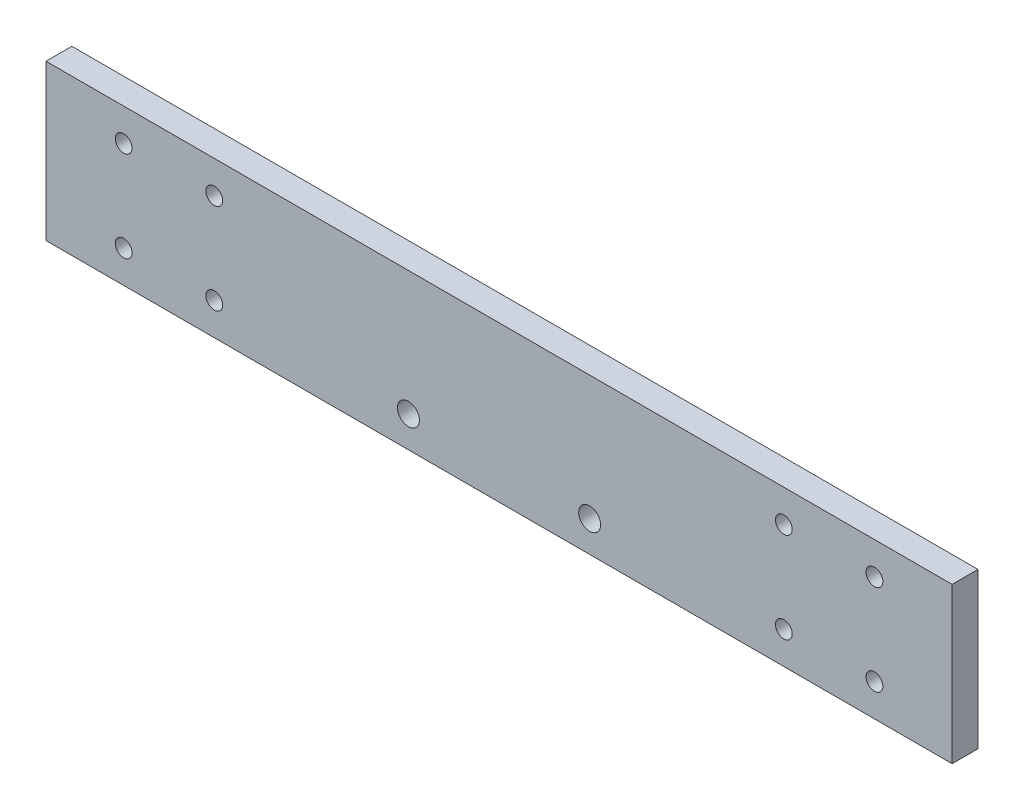
from build123d import *

# Parameters (mm, degrees)
SKETCH1_W           = 350
SKETCH1_H           = 60
SKETCH1_R           = 3.25
BOSS_EXTRUDE1_DEPTH = 10
M10_TAPPED_HOLE1_D  = 8.5


with BuildPart() as part:
    # Sketch1 → Boss-Extrude1 (new body)
    with BuildSketch(Plane.XY):
        with Locations((0, 30)):
            Rectangle(SKETCH1_W, SKETCH1_H)
        with Locations((-145, 47.5)):
            Circle(SKETCH1_R, mode=Mode.SUBTRACT)
        with Locations((-110, 47.5)):
            Circle(SKETCH1_R, mode=Mode.SUBTRACT)
        with Locations(Location((-110, 12.5, 0), (0, 0, 180))):
            Circle(SKETCH1_R, mode=Mode.SUBTRACT)
        with Locations(Location((-145, 12.5, 0), (0, 0, 180))):
            Circle(SKETCH1_R, mode=Mode.SUBTRACT)
        with Locations((110, 12.5)):
            Circle(SKETCH1_R, mode=Mode.SUBTRACT)
        with Locations((145, 12.5)):
            Circle(SKETCH1_R, mode=Mode.SUBTRACT)
        with Locations(Location((110, 47.5, 0), (0, 0, 180))):
            Circle(SKETCH1_R, mode=Mode.SUBTRACT)
        with Locations(Location((145, 47.5, 0), (0, 0, 180))):
            Circle(SKETCH1_R, mode=Mode.SUBTRACT)
    extrude(amount=BOSS_EXTRUDE1_DEPTH)

    # M10 Tapped Hole1 (through all)
    with Locations(Plane.XY.offset(10)):
        with Locations((-35, 12), (35, 12)):
            Hole(M10_TAPPED_HOLE1_D / 2)


solid = part.part
